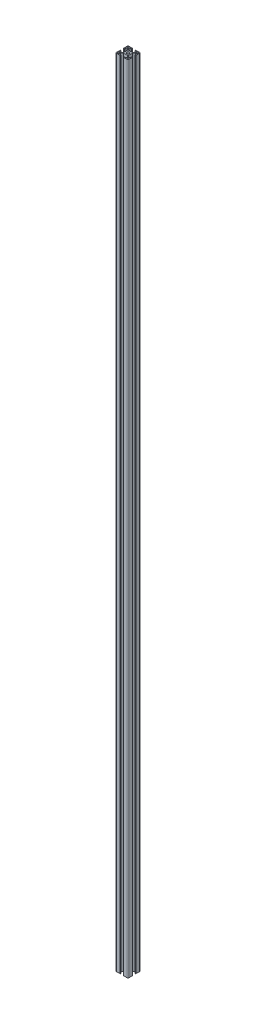
from build123d import *

# Parameters (mm, degrees)
SKETCH_1_R      = 2.1
SKETCH_1_R_2    = 3.4
EXTRUDE_1_DEPTH = 1940


with BuildPart() as part:
    # 草图1 → 拉伸1 (new body)
    with BuildSketch(Plane(origin=(0, 0, 0), x_dir=(1, 0, 0), z_dir=(0, 1, 0))):
        with BuildLine():
            Line((6.75, -28), (11, -28))
            Line((11, -28), (11, -30))
            Line((11, -30), (2, -30))
            ThreePointArc((2, -30), (0.585786438, -29.414213562), (0, -28))
            Line((0, -28), (0, -19))
            Line((0, -19), (2, -19))
            Line((2, -19), (2, -23.25))
            Line((2, -23.25), (5.335785999, -23.25))
            Line((5.335785999, -23.25), (9, -19.585785999))
            Line((9, -19.585785999), (9, -10.414214001))
            Line((9, -10.414214001), (5.335785999, -6.75))
            Line((5.335785999, -6.75), (2, -6.75))
            Line((2, -6.75), (2, -11))
            Line((2, -11), (0, -11))
            Line((0, -11), (0, -2))
            ThreePointArc((0, -2), (0.585786438, -0.585786438), (2, 0))
            Line((2, 0), (11, 0))
            Line((11, 0), (11, -2))
            Line((11, -2), (6.75, -2))
            Line((6.75, -2), (6.75, -5.335785999))
            Line((6.75, -5.335785999), (10.414214001, -9))
            Line((10.414214001, -9), (19.585785999, -9))
            Line((19.585785999, -9), (23.25, -5.335785999))
            Line((23.25, -5.335785999), (23.25, -2))
            Line((23.25, -2), (19, -2))
            Line((19, -2), (19, 0))
            Line((19, 0), (28, 0))
            ThreePointArc((28, 0), (29.414213562, -0.585786438), (30, -2))
            Line((30, -2), (30, -11))
            Line((30, -11), (28, -11))
            Line((28, -11), (28, -6.75))
            Line((28, -6.75), (24.664214001, -6.75))
            Line((24.664214001, -6.75), (21, -10.414214001))
            Line((21, -10.414214001), (21, -19.585785999))
            Line((21, -19.585785999), (24.664214001, -23.25))
            Line((24.664214001, -23.25), (28, -23.25))
            Line((28, -23.25), (28, -19))
            Line((28, -19), (30, -19))
            Line((30, -19), (30, -28))
            ThreePointArc((30, -28), (29.414213562, -29.414213562), (28, -30))
            Line((28, -30), (19, -30))
            Line((19, -30), (19, -28))
            Line((19, -28), (23.25, -28))
            Line((23.25, -28), (23.25, -24.664214001))
            Line((23.25, -24.664214001), (19.585785999, -21))
            Line((19.585785999, -21), (10.414214001, -21))
            Line((10.414214001, -21), (6.75, -24.664214001))
            Line((6.75, -24.664214001), (6.75, -28))
        make_face()
        with Locations(Location((3.375, -26.625, 0), (0, 0, 270))):
            Circle(SKETCH_1_R, mode=Mode.SUBTRACT)
        with Locations(Location((26.625, -26.625, 0), (0, 0, 270))):
            Circle(SKETCH_1_R, mode=Mode.SUBTRACT)
        with Locations(Location((15, -15, 0), (0, 0, 270))):
            Circle(SKETCH_1_R_2, mode=Mode.SUBTRACT)
        with Locations(Location((3.375, -3.375, 0), (0, 0, 270))):
            Circle(SKETCH_1_R, mode=Mode.SUBTRACT)
        with Locations(Location((26.625, -3.375, 0), (0, 0, 270))):
            Circle(SKETCH_1_R, mode=Mode.SUBTRACT)
    extrude(amount=EXTRUDE_1_DEPTH)


solid = part.part
